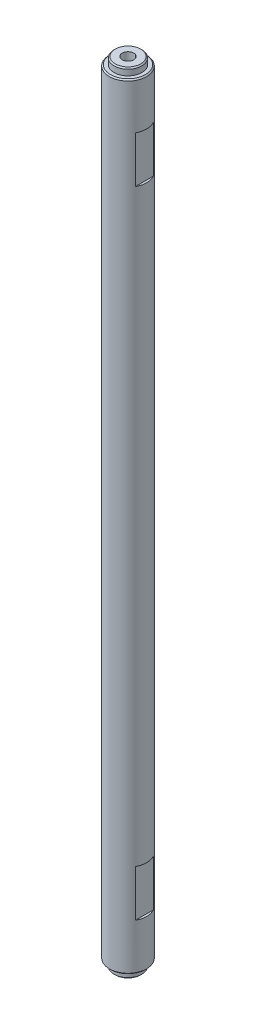
from build123d import *

# Parameters (mm, degrees)
SKETCH1_R             = 8
BOSS_EXTRUDE1_DEPTH   = 166.5
SKETCH2_R             = 6
BOSS_EXTRUDE2_DEPTH   = 3
CHAMFER1_SIZE         = 0.5
CUT_EXTRUDE2_START    = -40
CUT_EXTRUDE2_DEPTH    = 20
M6_TAPPED_HOLE1_D     = 5
M6_TAPPED_HOLE1_DEPTH = 17
M6_TAPPED_HOLE1_TIP   = 1.502151548
CHAMFER2_SIZE         = 0.5
BOSS_EXTRUDE3_START   = 3
SKETCH6_R             = 6
BOSS_EXTRUDE3_DEPTH   = 3
CHAMFER3_SIZE         = 0.5
M6_TAPPED_HOLE2_D     = 5
M6_TAPPED_HOLE2_DEPTH = 17
M6_TAPPED_HOLE2_TIP   = 1.502151548


with BuildPart() as part:
    # Sketch1 → Boss-Extrude1 (new, symmetric)
    with BuildSketch(Plane(origin=(0, 0, 0), x_dir=(1, 0, 0), z_dir=(0, 1, 0))):
        with Locations(Location((0, 0, 0), (0, 0, 270))):
            Circle(SKETCH1_R)
    extrude(amount=BOSS_EXTRUDE1_DEPTH, both=True)

    # Sketch2 → Boss-Extrude2 (add)
    with BuildSketch(Plane.XZ.offset(166.5)):
        with Locations(Location((0, 0, 0), (0, 0, 90))):
            Circle(SKETCH2_R)
    extrude(amount=BOSS_EXTRUDE2_DEPTH)

    # Chamfer1
    chamfer1_edges = [part.edges().sort_by_distance(p)[0] for p in [
        (0, -166.5, -8),
        (0, -169.5, -6),
    ]]
    chamfer(chamfer1_edges, length=CHAMFER1_SIZE)

    # Sketch3 → Cut-Extrude2 (cut)
    with BuildSketch(Plane.XZ.offset(166.5).offset(CUT_EXTRUDE2_START)):
        with BuildLine():
            Line((-7, 3.872983346), (-7, -3.872983346))
            ThreePointArc((-7, -3.872983346), (-8, 0), (-7, 3.872983346))
        make_face()
        with BuildLine():
            Line((7, 3.872983346), (7, -3.872983346))
            ThreePointArc((7, -3.872983346), (8, 0), (7, 3.872983346))
        make_face()
    cut_extrude2 = extrude(amount=CUT_EXTRUDE2_DEPTH, mode=Mode.SUBTRACT)

    # M6 Tapped Hole1
    with Locations(Plane.XZ.offset(169.5)):
        with Locations((0, 0)):
            Hole(M6_TAPPED_HOLE1_D / 2, depth=M6_TAPPED_HOLE1_DEPTH)
            with Locations((0, 0, -(M6_TAPPED_HOLE1_DEPTH + M6_TAPPED_HOLE1_TIP / 2))):  # 118° drill point
                Cone(0, M6_TAPPED_HOLE1_D / 2, M6_TAPPED_HOLE1_TIP, mode=Mode.SUBTRACT)

    # Chamfer2
    chamfer2_edges = [part.edges().sort_by_distance(p)[0] for p in [
        (0, 166.5, -8),
    ]]
    chamfer(chamfer2_edges, length=CHAMFER2_SIZE)

    # Sketch6 → Boss-Extrude3 (add)
    with BuildSketch(Plane(origin=(0, 166.5, 0), x_dir=(1, 0, 0), z_dir=(0, 1, 0)).offset(BOSS_EXTRUDE3_START)):
        with Locations(Location((0, 0, 0), (0, 0, 270))):
            Circle(SKETCH6_R)
    extrude(amount=-BOSS_EXTRUDE3_DEPTH)

    # Chamfer3
    chamfer3_edges = [part.edges().sort_by_distance(p)[0] for p in [
        (0, 169.5, -6),
    ]]
    chamfer(chamfer3_edges, length=CHAMFER3_SIZE)

    # M6 Tapped Hole2
    with Locations(Plane(origin=(0, 169.5, 0), x_dir=(-1, 0, 0), z_dir=(0, 1, 0))):
        with Locations((0, 0)):
            Hole(M6_TAPPED_HOLE2_D / 2, depth=M6_TAPPED_HOLE2_DEPTH)
            with Locations((0, 0, -(M6_TAPPED_HOLE2_DEPTH + M6_TAPPED_HOLE2_TIP / 2))):  # 118° drill point
                Cone(0, M6_TAPPED_HOLE2_D / 2, M6_TAPPED_HOLE2_TIP, mode=Mode.SUBTRACT)

    # Mirror1: Cut-Extrude2 across plane
    add(cut_extrude2.mirror(Plane.ZX), mode=Mode.SUBTRACT)


solid = part.part
